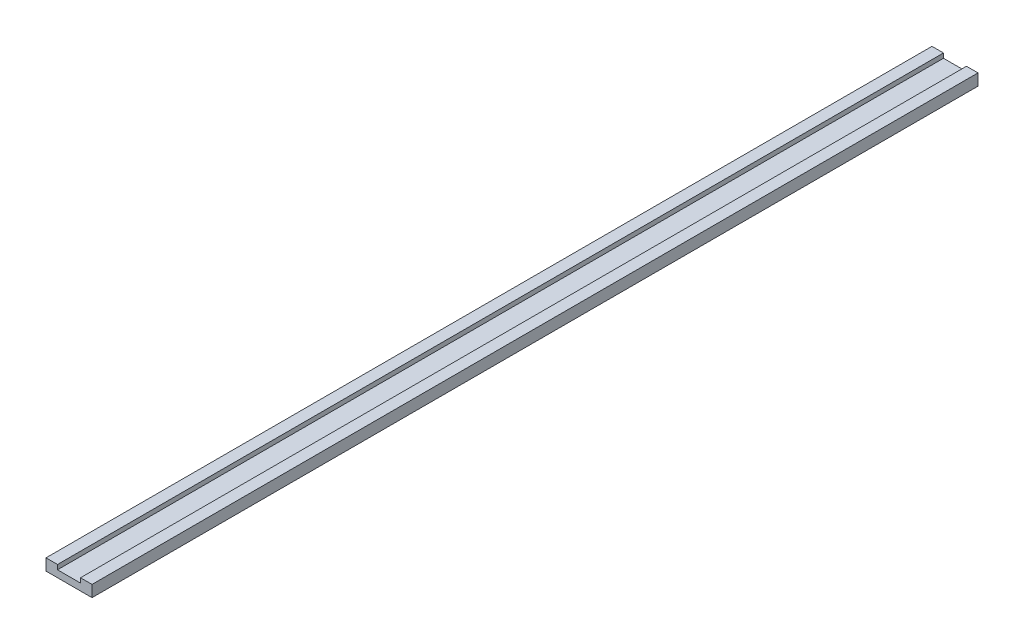
SolidWorks part; units mm, degrees
ref_plane "Front Plane" through (0, 0, 0) normal (0, 0, 1) x (1, 0, 0)
ref_plane "Top Plane" through (0, 0, 0) normal (0, 1, 0) x (1, 0, 0)
ref_plane "Right Plane" through (0, 0, 0) normal (1, 0, 0) x (0, 0, -1)
other "Configuration Table"
sketch "Sketch1" plane through (0, 0, 0) normal (0, 0, 1) x (1, 0, 0)
  line L0 (5, 5) -> (5, 3)
  line L1 (0, 0) -> (20, 0)
  line L2 (0, 0) -> (0, 5)
  line L3 (0, 5) -> (5, 5)
  line L4 (20, 0) -> (20, 5)
  line L5 (5, 3) -> (15, 3)
  line L6 (15, 3) -> (15, 5)
  line L7 (15, 5) -> (20, 5)
  dimension "D1" = 20
  dimension "D2" = 5
  dimension "D3" = 10
  dimension "D4" = 5
  dimension "D5" = 2
extrude "Boss-Extrude1" add sketch "Sketch1" along normal blind 385
